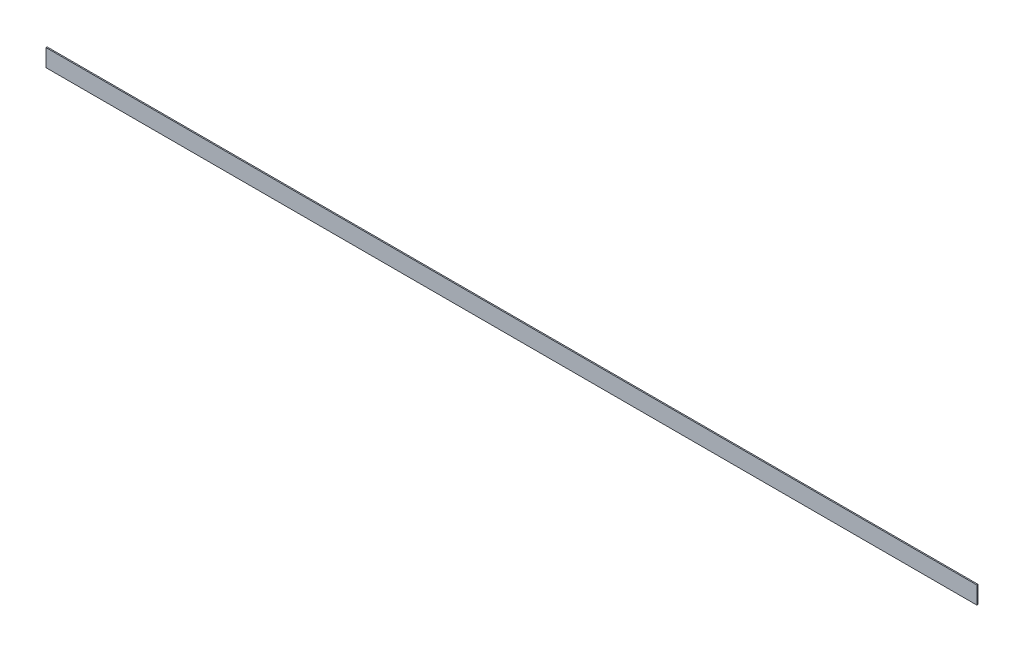
SolidWorks part; units mm, degrees
ref_plane "Front Plane" through (0, 0, 0) normal (0, 0, 1) x (1, 0, 0)
ref_plane "Top Plane" through (0, 0, 0) normal (0, 1, 0) x (1, 0, 0)
ref_plane "Right Plane" through (0, 0, 0) normal (1, 0, 0) x (0, 0, -1)
sketch "Sketch1" plane through (0, 0, 0) normal (0, 0, 1) x (1, 0, 0)
  line L1 (-8000, 150) -> (8000, 150)
  line L2 (-8000, 150) -> (-8000, -150)
  line L3 (-8000, -150) -> (8000, -150)
  line L4 (8000, 150) -> (8000, -150)
  line L5 (-8000, 150) -> (8000, -150) construction
  line L6 (-8000, -150) -> (8000, 150) construction
  point P0 (0, 0)
  dimension "D1" = 16000
  dimension "D2" = 300
extrude "Boss-Extrude1" add sketch "Sketch1" along normal blind 20
